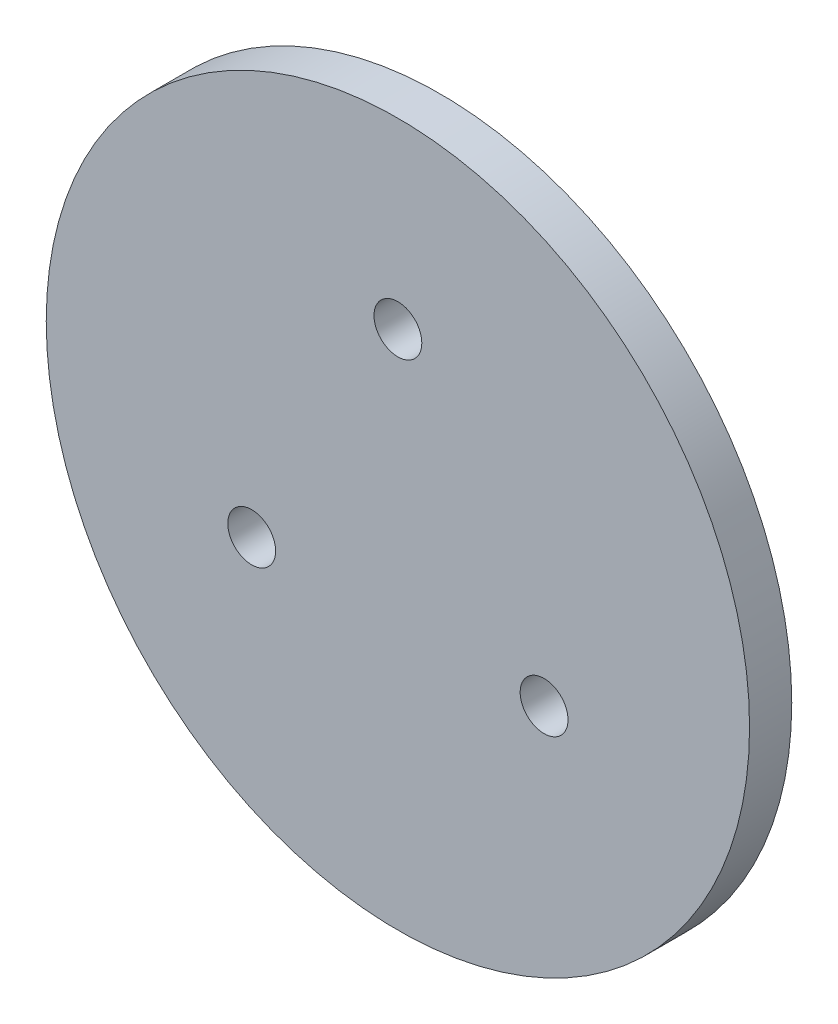
from build123d import *

# Parameters (mm, degrees)
SKETCH1_R           = 125
SKETCH1_R_2         = 8.5
BOSS_EXTRUDE1_DEPTH = 7.5


with BuildPart() as part:
    # Sketch1 → Boss-Extrude1 (new, symmetric)
    with BuildSketch(Plane.XY):
        Circle(SKETCH1_R)
        with Locations((0, 60)):
            Circle(SKETCH1_R_2, mode=Mode.SUBTRACT)
        with Locations((51.961524227, -30)):
            Circle(SKETCH1_R_2, mode=Mode.SUBTRACT)
        with Locations((-51.961524227, -30)):
            Circle(SKETCH1_R_2, mode=Mode.SUBTRACT)
    extrude(amount=BOSS_EXTRUDE1_DEPTH, both=True)


solid = part.part
